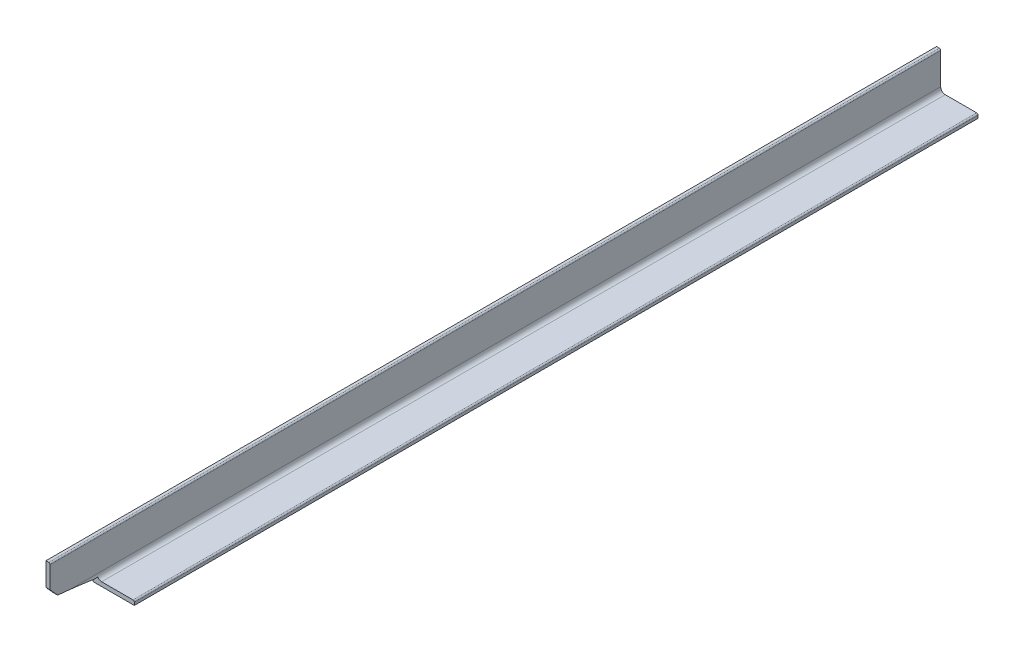
from build123d import *

# Parameters (mm, degrees)
GBT706_2008_050_5_1_DEPTH = 1073.5
CUT_EXTRUDE_1_REACH       = 1077.826


with BuildPart() as part:
    # Sketch1 → Gbt706-2008 热轧等边角钢 050×5(1) (new body)
    with BuildSketch(Plane.YX):
        with BuildLine():
            Line((0, 0), (0, 50))
            Line((0, 50), (3.333333333, 50))
            ThreePointArc((3.333333333, 50), (4.511844635, 49.511844635), (5, 48.333333333))
            Line((5, 48.333333333), (5, 10.5))
            ThreePointArc((5, 10.5), (6.610912703, 6.610912703), (10.5, 5))
            Line((10.5, 5), (48.333333333, 5))
            ThreePointArc((48.333333333, 5), (49.511844635, 4.511844635), (50, 3.333333333))
            Line((50, 3.333333333), (50, 0))
            Line((50, 0), (0, 0))
        make_face()
    extrude(amount=GBT706_2008_050_5_1_DEPTH)

    # 草图3 → 切除-拉伸1 (cut, up to next)
    with BuildSketch(Plane.ZY, mode=Mode.PRIVATE) as cut_extrude_1_sk1:
        Polygon((-56.5, 0), (-56.5, 7.501394609), (-52.022642316, 7.501394609), (-8.954715367, 12.028016136), (0, 21.973235089), (20, 21.973235089), (20, -8.026764911), (-56.5, -8.026764911), align=None)
    cut_extrude_1_tool1 = extrude(cut_extrude_1_sk1.sketch, amount=-CUT_EXTRUDE_1_REACH, mode=Mode.PRIVATE) & part.part
    add(cut_extrude_1_tool1.solids().sort_by_distance((0, 3.560964, -12.87534))[0], mode=Mode.SUBTRACT)


solid = part.part
